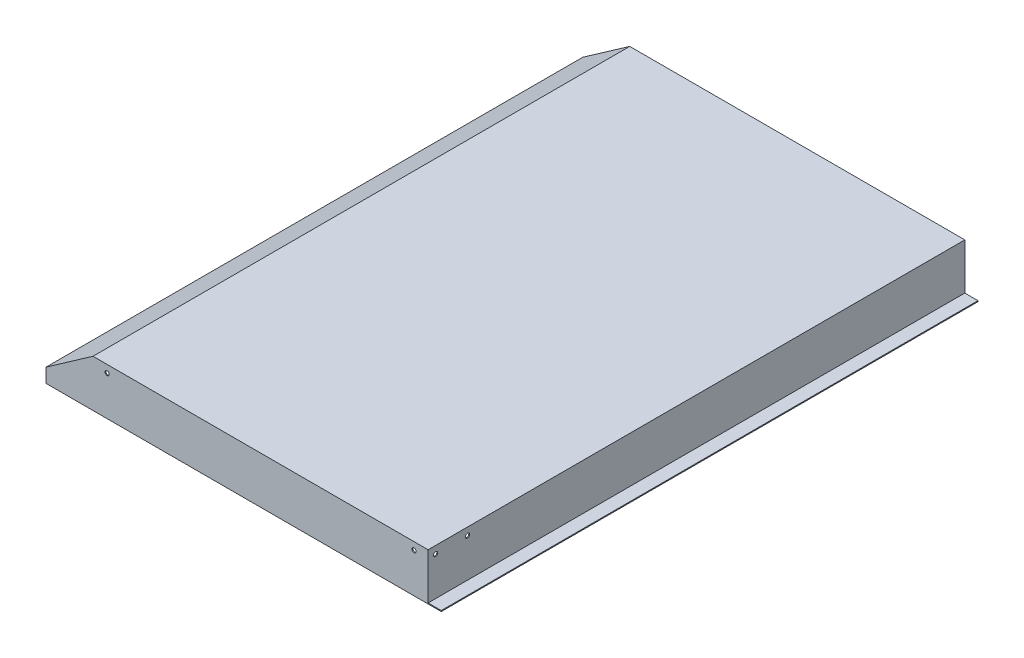
from build123d import *

# Parameters (mm, degrees)
EXTRUDE_1_DEPTH     = 571
SHELL_1_T           = -2
SKETCH_2_W          = 30
SKETCH_2_H          = 1142
EXTRUDE_2_DEPTH     = 2
SKETCH_3_R          = 4.5
CUT_EXTRUDE_1_DEPTH = 1175
EXTRUDE_3_DEPTH     = 2
SKETCH_6_R          = 4.5
CUT_EXTRUDE_2_DEPTH = 2
SKETCH_7_R          = 4.5
CUT_EXTRUDE_3_DEPTH = 10


with BuildPart() as part:
    # 草图1 → 凸台-拉伸1 (new, symmetric)
    with BuildSketch(Plane.XY):
        Polygon((0, 0), (-813, 0), (-813, 30), (-713.029639528, 100), (0, 100), align=None)
    extrude(amount=EXTRUDE_1_DEPTH, both=True)

    # 抽壳1
    shell_1_openings = [part.faces().sort_by_distance(p)[0] for p in [
        (-406.5, 0, 0),
    ]]
    offset(amount=SHELL_1_T, openings=shell_1_openings, kind=Kind.INTERSECTION)

    # 草图2 → 凸台-拉伸2 (add)
    with BuildSketch(Plane.XZ):
        with Locations((13, 0)):
            Rectangle(SKETCH_2_W, SKETCH_2_H)
    extrude(amount=-EXTRUDE_2_DEPTH)

    # 草图3 → 切除-拉伸1 (cut)
    with BuildSketch(Plane.XY.offset(571)):
        with Locations((-683.029639528, 84)):
            Circle(SKETCH_3_R)
        with Locations((-30, 84)):
            Circle(SKETCH_3_R)
    extrude(amount=-CUT_EXTRUDE_1_DEPTH, mode=Mode.SUBTRACT)

    # 草图5 → 凸台-拉伸3 (add)
    with BuildSketch(Plane.XZ):
        Polygon((-783, 541), (0, 541), (0, 571), (-813, 571), (-813, -571), (0, -571), (0, -541), (-783, -541), align=None)
    extrude(amount=-EXTRUDE_3_DEPTH)

    # 草图6 → 切除-拉伸2 (cut)
    with BuildSketch(Plane.XZ):
        with Locations((-797, 541)):
            Circle(SKETCH_6_R)
        with Locations((-797, -541)):
            Circle(SKETCH_6_R)
        with Locations((-797, 0)):
            Circle(SKETCH_6_R)
    extrude(amount=-CUT_EXTRUDE_2_DEPTH, mode=Mode.SUBTRACT)

    # 草图7 → 切除-拉伸3 (cut)
    with BuildSketch(Plane(origin=(0, 0, 0), x_dir=(0, 0, -1), z_dir=(1, 0, 0))):
        with Locations((-555, 84)):
            Circle(SKETCH_7_R)
        with Locations((-487, 84)):
            Circle(SKETCH_7_R)
    extrude(amount=-CUT_EXTRUDE_3_DEPTH, mode=Mode.SUBTRACT)


solid = part.part
